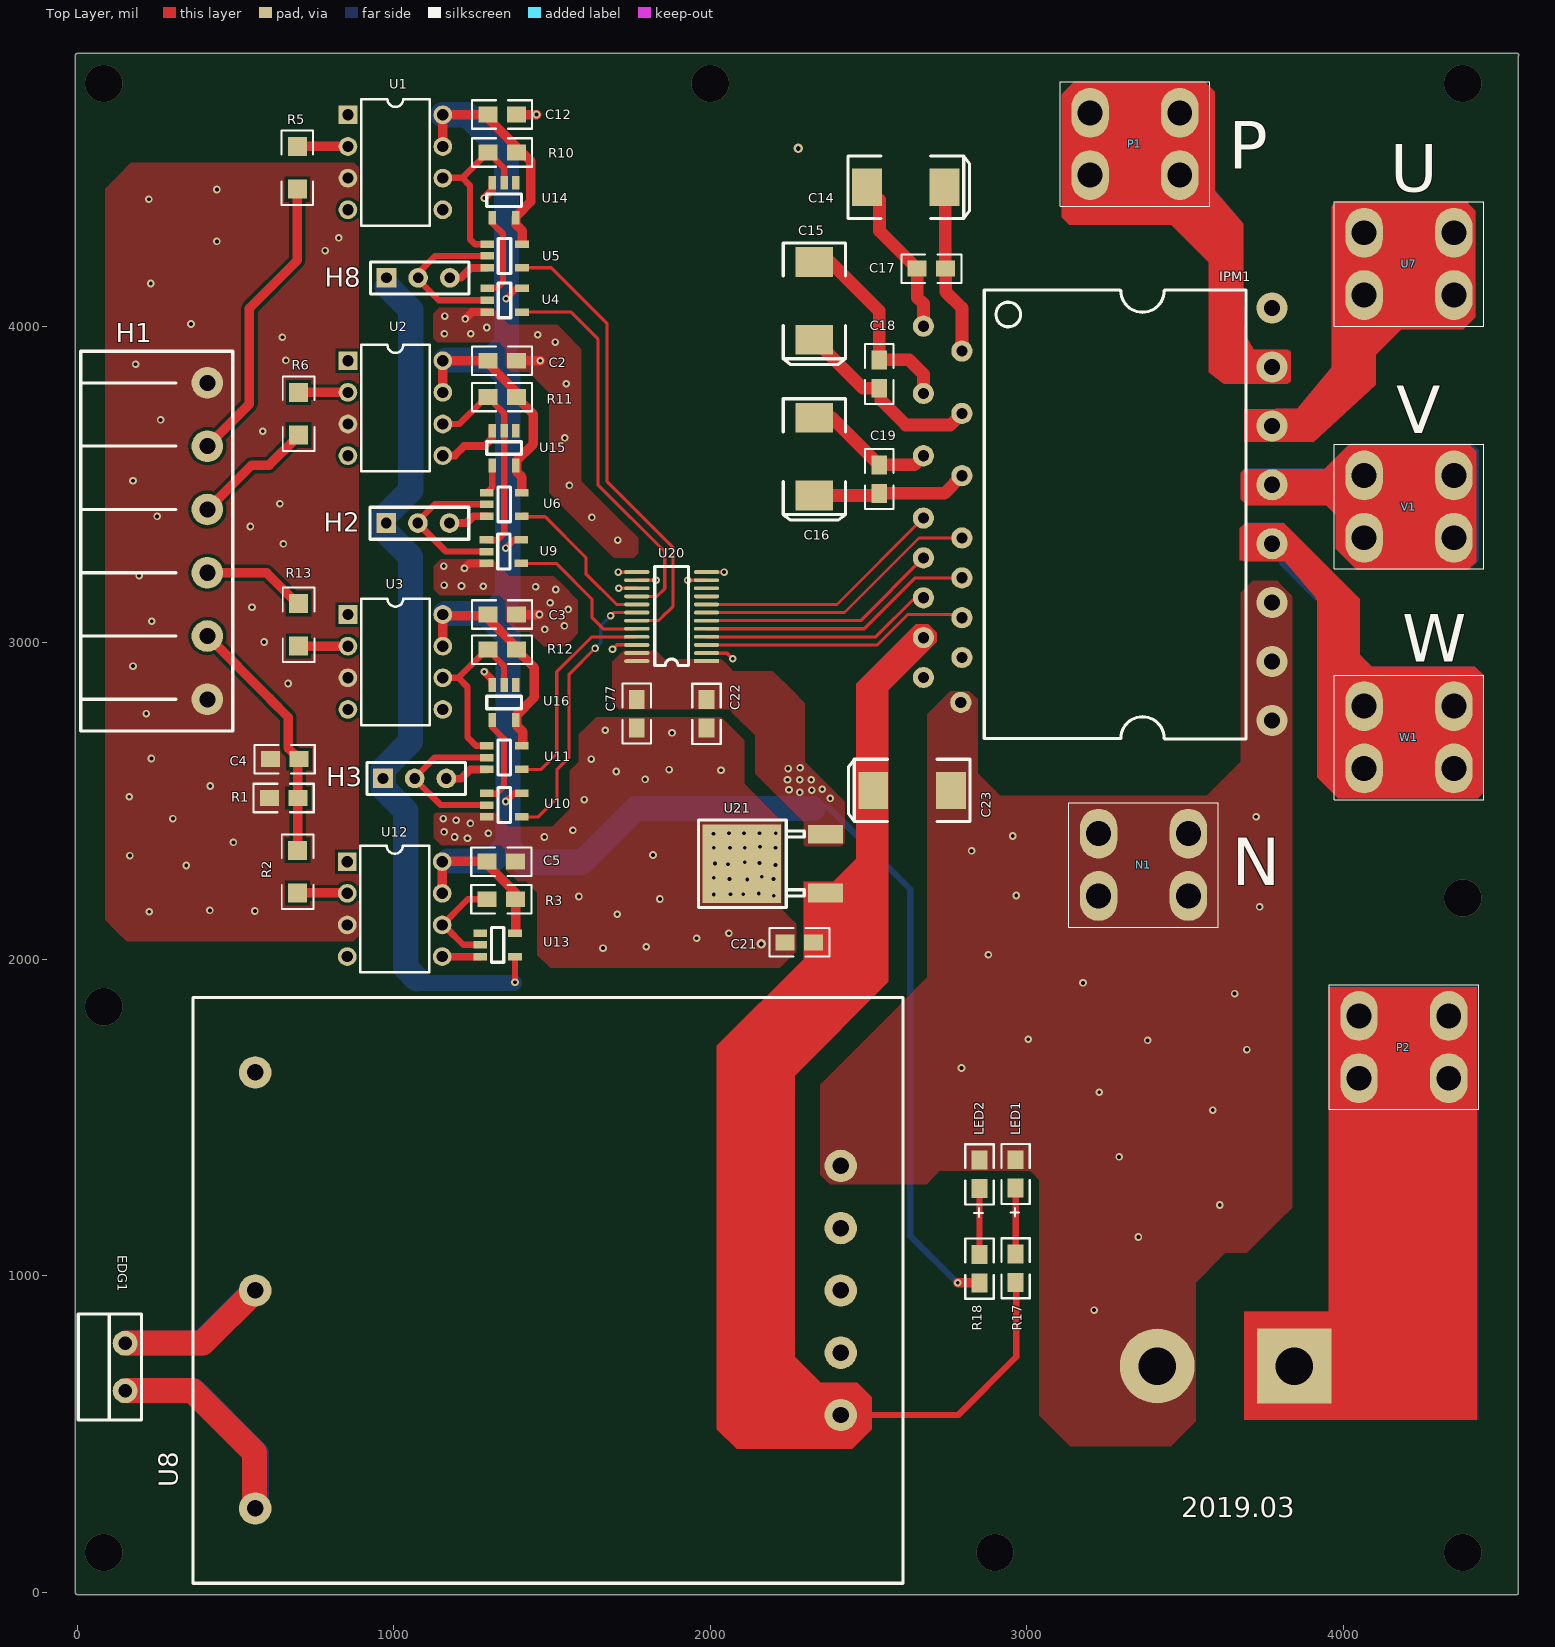
[diagram p0: Top Layer view]
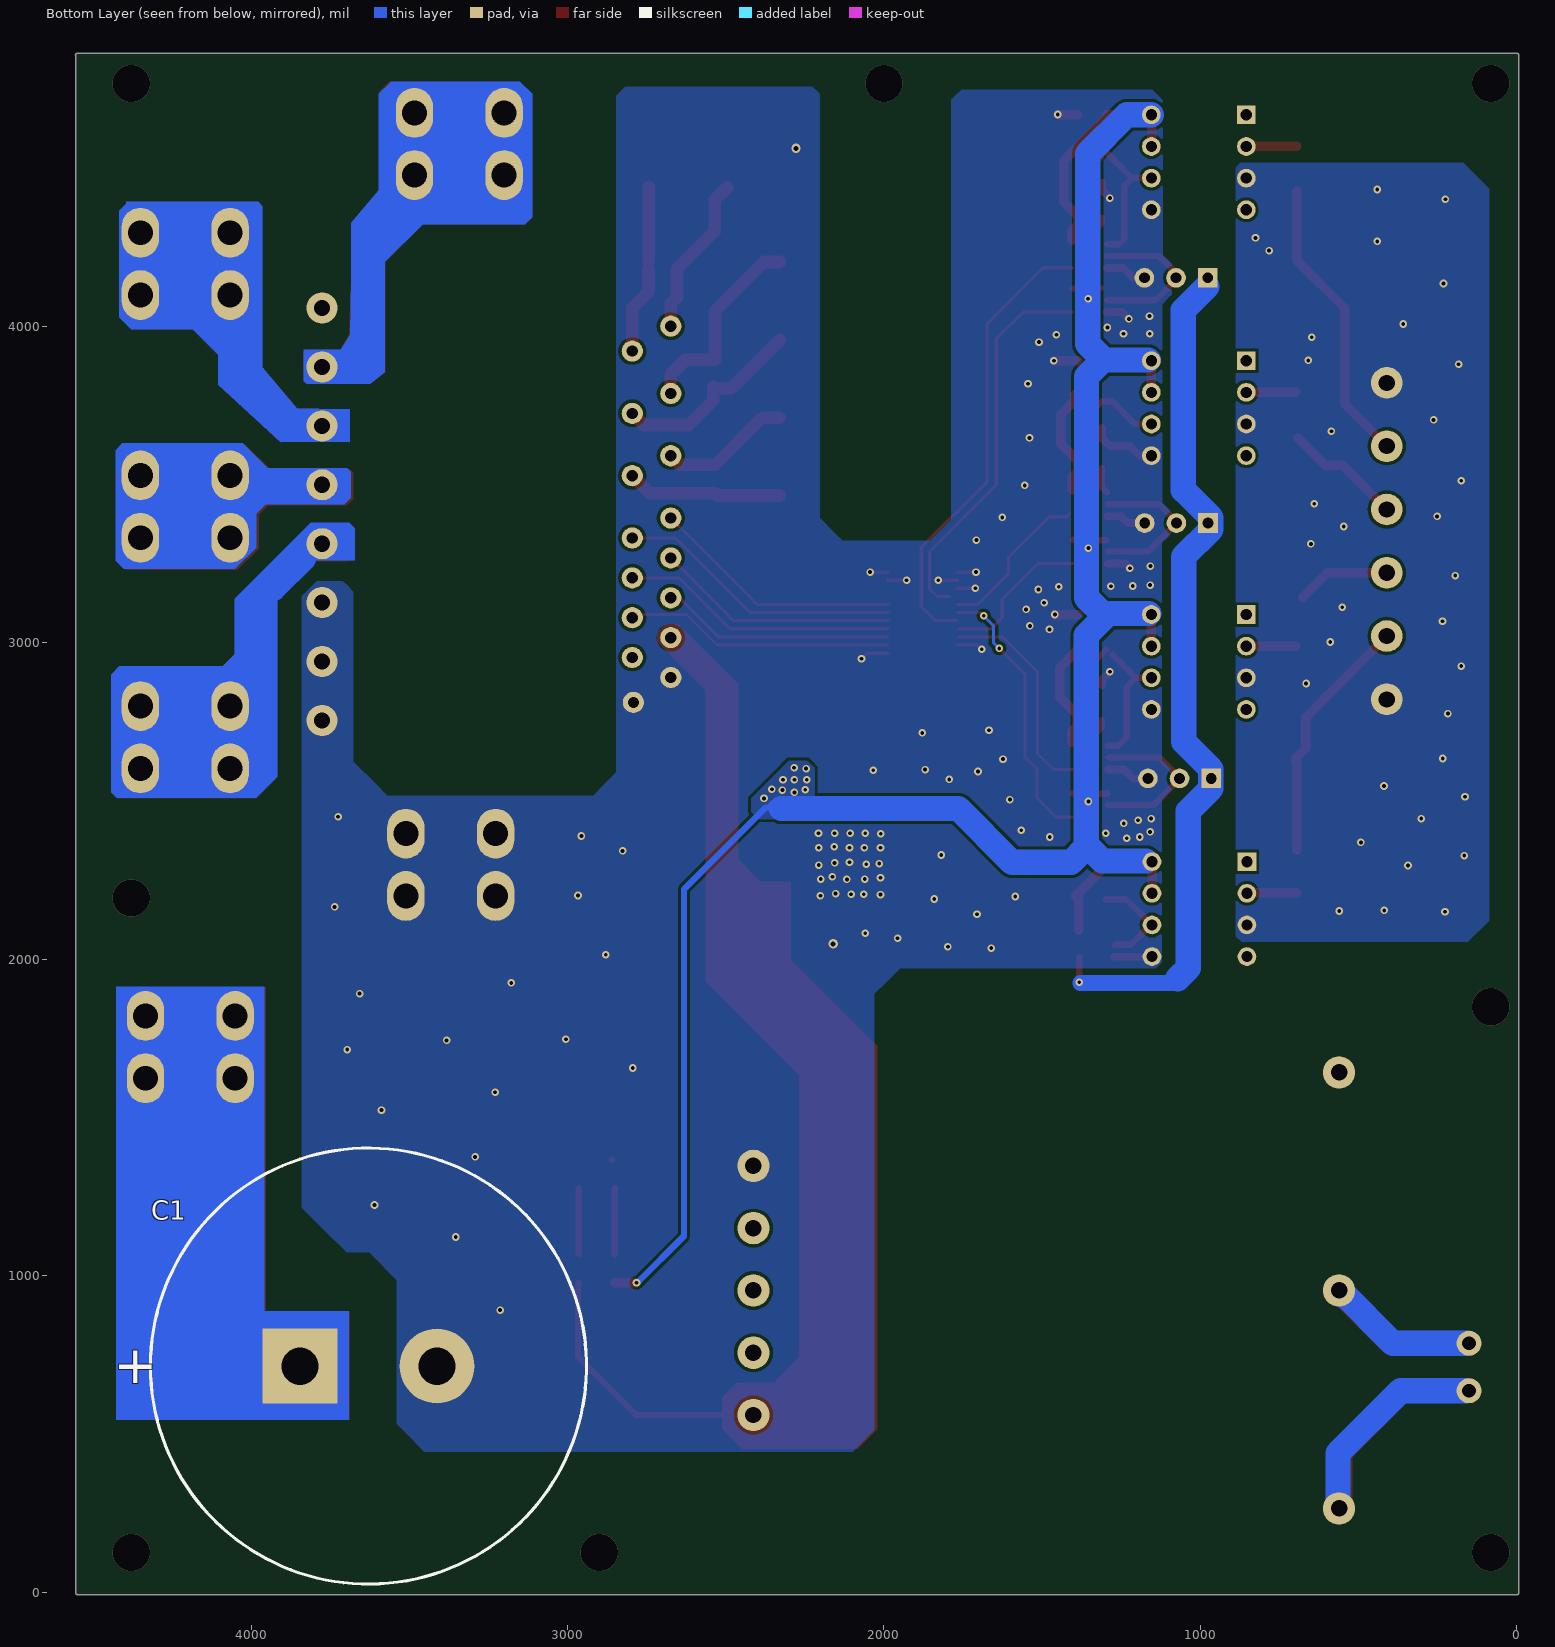
[diagram p1: Bottom Layer view, seen from below]
# Altium PCB MISC81124.PcbDoc
Units mil, origin at the board's own origin, x right, y up, seen from the top; angles counter-clockwise.
Board outline 4561.03 x 4870.03 mil, 2 copper layers (Top Layer, Bottom Layer); 58 components, 50 nets, 240 pads, 164 vias.

## Layer stack, top to bottom (the 12.6 mil dielectric is the usual default, probably not edited)
Top Layer: signal copper 1.4
Dielectric: dielectric 12.6, FR-4, Dk 4.8
Bottom Layer: signal copper 1.4

## Board outline
-6.01,-3 ccw(c-1,-3) -1,-8.01 4547,-8.01 ccw(c4547,-3) 4548,-7.91 ccw(c4549,-3) 4554.01,-3 4554.01,4853.99 ccw(c4550,4857) 4555.01,4857 ccw(c4550,4857) 4550,4862.02 -1,4862.02 ccw(c-1,4857) -6.01,4857

## Design rules (kind name [scope] priority, off if disabled: settings)
Clearance [All] p1: gap=10
ComponentClearance [All] p1 off: gap=10 collisioncheckmode=3 verticalgap=10 showdistances=FALSE
FabricationTestPointUsage TestPointUsage [All] p1: valid=0 allowmultiple=FALSE
FabricationTestpoint Testpoint [(IsPad And (OnTopLayer Or OnBottomLayer))] p1: side=3 testpointundercomponent=TRUE minsize=40 maxsize=100 preferedsize=60 minholesize=0 maxholesize=40 preferedholesize=32 testpointgrid=1 allowsidetop=TRUE allowsidebottom=TRUE usegrid=TRUE gridtolerance=0.01
FanoutControl Fanout_LCC [All] p1 off: bgadir=Out bgaviamode=Centered fanoutstyle=Auto fanoutdirection=Alternating viagrid=1 // Protel DXP Scope 1 Expression Was: IsLCC   Fanout_LCC (Default Rule)
FanoutControl Fanout_BGA [All] p2 off: bgadir=Out bgaviamode=Centered fanoutstyle=Auto fanoutdirection=Alternating viagrid=1 // Protel DXP Scope 1 Expression Was: IsBGA   Fanout_BGA (Default Rule)
FanoutControl Fanout_SOIC [All] p3 off: bgadir=Out bgaviamode=Centered fanoutstyle=Auto fanoutdirection=Alternating viagrid=1 // Protel DXP Scope 1 Expression Was: IsSOIC   Fanout_SOIC (Default Rule)
FanoutControl Fanout_Default [All] p4: bgadir=Out bgaviamode=Centered fanoutstyle=Auto fanoutdirection=Alternating viagrid=1 // Fanout_Default (Default Rule)
FanoutControl Fanout_Small [All] p5 off: bgadir=Out bgaviamode=Centered fanoutstyle=Auto fanoutdirection=Alternating viagrid=1 // Protel DXP Scope 1 Expression Was: (CompPinCount < 5)   Fanout_Small (Default Rule)
Height [All] p1 off: minheight=0 maxheight=1000 prefheight=500
HoleSize [All] p1: absolutevalues=TRUE maxlimit=150 minlimit=6 maxpercent=80.000 minpercent=20.000
MinimumSolderMaskSliver [All] p1: minsoldermaskwidth=0
PlaneConnect [All] p1: planeconnectstyle=Direct reliefexpansion=20 reliefentries=4 reliefconductorwidth=10 reliefairgap=10
PolygonConnect [All] p1: connectstyle=Direct reliefconductorwidth=75 reliefentries=4 polygonreliefangle="90 Angle"
RoutingVias [All] p1: holewidth=12 width=24 viastyle="Through Hole" minholewidth=12 minwidth=24 maxholewidth=12 maxwidth=24
SilkToSilkClearance [All] p1: silktosilkclearance=0
SilkscreenOverComponentPads [IsPad] p1 off: minsilkscreentomaskgap=10 // Protel DXP Scope 1 Expression Was: IsPad
SolderMaskExpansion [All] p1: expansion=4
Width [All] p1: maxlimit=99 minlimit=10 preferedwidth=11.81
14 further rules are at their usual default settings.

## Components (designator, comment, footprint, x,y, rotation, side; value= is the part's Value field where it differs from the comment)
C1 "450V" ElecCap_450V 3629,714 r180 bottom
C2 "0.1uF" 0805 1387,3891 r180 top
C3 "0.1uF" 0805 1387,3089 r180 top
C4 "30pF" 0805 610,2632 r0 top
C5 "0.1uF" 0805 1385,2308 r180 top
C12 "0.1uF" 0805 1387,4669 r180 top
C14 "22uF/35V" 7343_CASE-D 2618,4439 r0 top
C15 "22uF/35V" 7343_CASE-D 2329,4080 r270 top
C16 "22uF/35V" 7343_CASE-D 2329,3588 r270 top
C17 "0.1uF" 0805 2744,4182 r180 top
C18 "0.1uF" 0805 2534,3804 r90 top
C19 "0.1uF" 0805 2534,3472 r90 top
C21 "0.33uF" 0805 2237,2053 r0 top
C22 "0.01uF" 0805 1988,2730 r90 top
C23 "22uF/35V" 7343_CASE-D 2638,2533 r180 top
C77 "0.1uF" 0805 1768,2821 r270 top
EDG1 "EDG 2p" EDGCon_2p_3.81mm 151,786 r270 top
H1 "Header6" EDGCon_6P_5.08mm 411,3821 r270 top
H2 "Header3" PinHeader3_2.54mm 976,3378 r0 top
H3 "Header3" PinHeader3_2.54mm 966,2571 r0 top
H8 "Header3" PinHeader3_2.54mm 977,4153 r0 top
IPM1 "IKCM15F60GA" IKCM15F60GA 3692.77,2697 r90 top
LED1 "LED" 0805_LED 2965,1276 r90 top
LED2 "LED" 0805_LED 2851,1275 r90 top
N1 "PCBTerminator" PCBTerminator 3369,2298 r90 top
P1 "PCBTerminator" PCBTerminator 3342,4576 r90 top
P2 "PCBTerminator" PCBTerminator 4192,1722 r90 top
R1 "10k" 0805 607,2509 r0 top
R2 "500R" 1206 696,2209 r90 top
R3 "10k" 0805 1295,2189 r0 top
R5 "500R" 1206 695,4568 r270 top
R6 "500R" 1206 699,3791 r270 top
R10 "10k" 0805 1297,4549 r0 top
R11 "10k" 0805 1297,3776 r0 top
R12 "10k" 0805 1297,2978 r0 top
R13 "500R" 1206 699,2989 r90 top
R17 "10k" 0805 2965,1068 r270 top
R18 "3.3k" 0805 2851,1067 r270 top
U1 "6N137" DIP-8 855,4668 r0 top
U2 "6N137" DIP-8 855,3891 r0 top
U3 "6N137" DIP-8 855,3089 r0 top
U4 "SN74AHC1G08" SOT-23-5 1350,4082 r180 top
U5 "SN74AHC1G08" SOT-23-5 1350,4222 r180 top
U6 "SN74AHC1G08" SOT-23-5 1349,3437 r180 top
U7 "PCBTerminator" PCBTerminator 4208,4197 r90 top
U8 "YAS5-15-W" YAS5 1487.2,953.02 r180 top
U9 "SN74AHC1G08" SOT-23-5 1348,3288 r180 top
U10 "SN74AHC1G08" SOT-23-5 1349,2487 r180 top
U11 "SN74AHC1G08" SOT-23-5 1349,2637 r180 top
U12 "6N137" DIP-8 853,2308 r0 top
U13 "SN74AHC1G04" SOT-23-5 1328,2045 r180 top
U14 "SN74AHC1G04" SOT-23-5 1348.65,4398 r90 top
U15 "SN74AHC1G04" SOT-23-5 1348.65,3615 r90 top
U16 "SN74AHC1G04" SOT-23-5 1348.65,2811 r90 top
U20 "SN74LVC8T245" SN74LVC8T245_TSSOP24 1988,3223.13 r180 top
U21 "L78M05" TO-252-2(DPAK) 2364,2302 r0 top
V1 "PCBTerminator" PCBTerminator 4208,3430 r90 top
W1 "PCBTerminator" PCBTerminator 4208,2701 r90 top

## Footprints (in the part's own frame and the unit in brackets; to place one, negate y for a bottom-side part, rotate by r counter-clockwise, add the part's x,y. Pads: shape width x height; smd on the part's side, far side on the other; paste and mask are expansions set on the pad)
0805 [mil]
  rect 60x50 smd: 1(0,0) 2(90,0)
  silkscreen extent -50,-45 140,45
0805_LED [mil]
  rect 60x50 smd: A(0,0) K(90,0)
  silkscreen extent -90,-45 140,45
1206 [mil]
  rect 60x60 smd: 1(0,0) 2(135,0)
  silkscreen extent -50,-50 185,50
7343_CASE-D [mm]
  rect 2.4x3 smd: 1(3.12,0) 2(-3.12,0)
  silkscreen extent -4.65,-2.5 5.1,2.5
DIP-8 [mm]
  rect 1.5x1.5 hole 0.9: 1(0,0)
  round 1.5 hole 0.9: 2(0,-2.54) 3(0,-5.08) 4(0,-7.62) 5(7.62,-7.62) 6(7.62,-5.08) 7(7.62,-2.54) 8(7.62,0)
  silkscreen extent 1.06,-8.88 6.56,1.27
EDGCon_2p_3.81mm [mm]
  round 2 hole 1.1: 1(0,0) 2(3.81,0)
  silkscreen extent -2.34,-3.76 6.15,1.32
EDGCon_6P_5.08mm [mil]
  round 100 hole 51: 1(0,0) 2(200,0) 3(400,0) 4(600,0) 5(800,0) 6(1000,0)
  silkscreen extent -100,-400 1100,80
ElecCap_450V [mm] "820"
  rect 6x6 hole 3: 1(-5.5,0)
  round 6 hole 3: 2(5.5,0)
  silkscreen extent -17.5,-17.5 17.5,17.5
IKCM15F60GA [mm] "Infineon IPM"
  round 1.7 hole 0.9: 1(33.1,25.885) 2(31.1,22.793) 3(27.7,25.885) 4(26.1,22.793) 5(22.7,25.885) 6(21.1,22.793) 7(17.7,25.885) 8(16.1,22.793) 9(14.5,25.885) 10(12.9,22.793) 11(11.3,25.885) 12(9.7,22.793) 13(8.1,25.885) 14(6.507,22.793) 15(4.9,25.885) 16(2.9,22.885)
  round 2.5 hole 1.3: 17(1.45,-2.1) 18(6.18,-2.1) 19(10.91,-2.1) 20(15.64,-2.1) 21(20.37,-2.1) 22(25.1,-2.1) 23(29.83,-2.1) 24(34.56,-2.1)
  silkscreen extent -0.03,0 36,21
PCBTerminator [mm]
  oval 4x3 hole 2: 1(-2.5,3.6) 1(-2.5,-3.6) 1(2.5,3.6) 1(2.5,-3.6)
  silkscreen extent -5,-6 5,6
PinHeader3_2.54mm [mil]
  rect 62x62 hole 34: 1(0,0)
  round 62 hole 34: 2(100,0) 3(200,0)
  silkscreen extent -51,-51 261,50
SN74LVC8T245_TSSOP24 [mil]
  rect 80x12 smd: 1(0,281.49)
  oval 80x12 smd: 2(0,255.9) 3(0,230.31) 4(0,204.72) 5(0,179.13) 6(0,153.54) 7(0,127.95) 8(0,102.36) 9(0,76.77) 10(0,51.18) 11(0,25.59) 12(0,0) 13(220,0) 14(220,25.59) 15(220,51.18) 16(220,76.77) 17(220,102.36) 18(220,127.95) 19(220,153.54) 20(220,179.13) 21(220,204.72) 22(220,230.31) 23(220,255.9) 24(220,281.49)
  silkscreen extent 56,-18 163,295
SOT-23-5 [mm]
  rect 1.1x0.6 smd: 1(1.4,-0.95) 2(1.4,0) 3(1.4,0.95) 4(-1.4,0.95) 5(-1.4,-0.95)
  silkscreen extent -0.5,-1.4 0.5,1.4
TO-252-2(DPAK) [mm]
  rect 6.3x6.3 smd: 1(-6.7,0)
  rect 2.8x1.5 smd: 2(-0.004,2.361) 3(0,-2.361)
  silkscreen extent -10.2,-3.52 -1.7,3.5
YAS5 [mm]
  round 2.6 hole 1.321: 1(23.5,17.5) 2(23.5,0) 3(23.5,-17.5) 4(-23.5,-10) 5(-23.5,-5) 6(-23.5,0) 7(-23.5,5) 8(-23.5,10)
  silkscreen extent -28.5,-23.5 28.5,23.5

## Part data
C1: library part ELECTROCap, "Electrolytic Capacitor(Pin1 Positive)"
C2 C3 C4 C5 C12 C17 C18 C19 C21 C22 C77: library part CAP, "Capacitor"
C14 C15 C16 C23: library part TaCap_D, "TaCap_D"
N1 P1 P2 U7 V1 W1: "PCB terminal for high current"
R1 R2 R3 R5 R6 R10 R11 R12 R13 R17 R18: library part RES2
U1 U2 U3 U12: "High-speed optocoupler"
U4 U5 U6: "Single 2-Input Positive-AND Buffer"
U8: library part YAS5
U9 U10 U11 U13 U14 U15 U16: "Single Input Inverter"
U20: "TI SN74LVC8T245PWR"
U21: library part LM1085ISX-3.3

## Via types
v1: diameter 24, hole 12, Top Layer to Bottom Layer, 154 vias
v2: diameter 118.11, hole 118.11, Top Layer to Bottom Layer, 8 vias
v3: diameter 30, hole 15, Top Layer to Bottom Layer, tented both sides, 2 vias

## Nets (pads, with @x,y where several pads share a name; then routed paths per layer and width w, separated by ;. In a path a pad name is that pad's centre, name@x,y a point inside that pad or via, vN(x,y) a via of type N, cw(c..) or ccw(c..) an arc to the next point about the centre after c; other vN are vias at no path point)
+5V_IPM: C2.2 C3.2 C5.2 C12.2 C22.2 C77.1 R3.2 R10.2 R11.2 R12.2 R18.2 U1.7 U1.8 U2.7 U2.8 U3.7 U3.8 U4.5 U5.5 U6.5 U9.5 U10.5 U11.5 U12.7 U12.8 U13.5 U14.5 U15.5 U16.5 U20.1 U20.23 U20.24 U21.2 | length 8699.7
  Top Layer w20: v1(1354,2498) 1380.4,2524.4 U10.5 ; v1(1354,3299) 1380.4,3325.4 U9.5 ; v1(1355,4087) 1387.4,4119.4 U4.5
  Top Layer w30: U12.7 U12.8 1153,2310 1293,2310 1297,2306 1297,2297 R3.2@1395,2199 ; U1.7@1154,4579 1154,4662 1164,4672 1167,4669 C12.2 C12.2@1297,4668.64 ; U3.7 1155,3082 1158,3085 C3.2@1283,3085 ; U2.7 U2.8@1155,3884 ; U2.8@1160,3891 C2.2 1297,3883 R11.2@1398,3782 ; C3.2@1283,3083 1291,3083 1387,2987 R12.2 1444,2921 1444,2827 1389,2772 1389,2737 1407,2719 U11.5@1407,2686 ; C12.2@1289,4668 1289,4666 1432.5,4522.5 1432.5,4393.5 U14.5@1392,4353 ; U13.5@1385,2091 R3.2 ; U14.5 1386.06,4321.94 1406,4302 1406,4272 ; R11.2 1441,3722 1441,3628 1388,3575 1388,3540 1405,3523 U6.5@1405,3484 ; v1(2782,977) R18.2
  Bottom Layer w20: 2345,2479 2374,2479 2632,2221 2632,1125 v1@2780,977
  Bottom Layer w50: U12.8@1157,2310 U12.8@1172,2310 ; U3.8@1160,3090 U3.8@1163,3090 ; U2.8@1160,3893 U2.8@1165,3893 ; 2325,2480 2343,2480
  Bottom Layer w80: U1.8 1233,4668 1356,4545 1356,3944 1305,3893 U2.8@1165,3893 ; U3.8@1163,3092 1292,3092 1361,3023 1361,2409 1361,2354 1409,2306 1595,2306 1765,2476 2325,2476 ; U12.8@1172,2310 1310,2310 1359,2359 ; 1308,3893 1360,3841 1360,3142 1310,3092
  other v1: 2379,2508 2283,2527 2321,2534 2249,2535 2354,2537 2244,2567 2283,2567 2319,2567 2246,2602 2284,2605
+15V_IPM: C21.2 C23.1 IPM1.13 R17.2 U8.8 U21.3 | length 1600.4
  Top Layer w20: U8.8@2421.07,568 U8.8 2783.32,559.32 2967,743 R17.2@2967,970 ; R17.2@2962,975 R17.2
  Top Layer w50: 2499,2362 2499,2841.24 IPM1.13
AC1: EDG1.2 U8.1 | length 1282.8
  Top Layer w80: EDG1.2@157,637 364,637 560,441 U8.1@560,265
  Bottom Layer w80: EDG1.2@161,636 368,636 565,439 U8.1@565,302
AC2: EDG1.1 U8.2 | length 940.7
  Top Layer w80: EDG1.1@155,787 392,787 ; 396,787 U8.2@561,952
  Bottom Layer w80: EDG1.1@154,786 391,786 U8.2@556,951
GND: C4.1 H1.1 H1.6 R1.1 U1.3 U2.3 U3.3 U12.3
  other v1: 227,2150 561,2152 419,2154 344,2296 166,2327 493,2369 302,2444 164,2513 420,2547 234,2634 218,2776 666,2871 176,2926 590,3002 235,3068 552,3112 195,3212 651,3312 547,3367 252,3399 640,3439 176,3512 586,3668 263,3704 184,3880 659,3892 648,3965 359,4007 232,4135 783,4239 441,4268 826,4279 226,4401 441,4432
IPM_N: C1.2 C2.1 C3.1 C5.1 C12.1 C21.1 C22.1 C23.2 C77.2 H2.3 H3.3 H8.3 IPM1.15 IPM1.16 IPM1.17 IPM1.18 IPM1.19 LED1.K LED2.K N1.1 U1.5 U2.5 U3.5 U4.3 U5.3 U6.3 U8.4 U9.3 U10.3 U11.3 U12.5 U13.3 U14.3 U15.3 U16.3 U20.2 U20.11 U20.12 U20.13 U20.14 U20.15 U20.22 U21.1 | length 1692.9
  Top Layer w11: v1(1691,2979) 1704.82,2992.82 U20.22 ; v1(1709.13,3223.13) U20.13 ; v1(1710.95,3171.95) U20.15 ; U20.14 v1(1828.46,3197.54) ; v1(1928.54,3197.54) U20.11 ; U20.2 2052.77,2967.23 v1(2071,2949) ; U20.12 v1(2043.87,3223.13)
  Top Layer w20: LED2.K@2858,1366 LED2.K@2859,1365
  Top Layer w25: U2.5@1142,3592 1193,3592 1222,3621 1286,3621 1311.25,3646.25 U15.3 ; H3.3@1148,2570 1212,2570 1241.6,2599.6 U11.3 ; U12.5@1164.4,2007.6 U13.3 ; H8.3@1173,4154 1213,4154 1243.6,4184.6 U5.3 ; H2.3@1174,3378 1230,3378 1251.6,3399.6 U6.3 ; v1(1223,3235) 1238.6,3250.6 U9.3 ; v1(1226,4023) 1247.6,4044.6 U4.3 ; v1(1286,2908) 1311.25,2882.75 U16.3 ; v1(1286,4405) 1311.25,4430.25 U14.3 ; U15.3@1311,3678 U15.3@1311.25,3677.75
  Top Layer w30: C3.1 v1(1460,3089) ; C2.1 v1(1463,3891) ; C12.1 v1(1451,4669)
  Bottom Layer w60: IPM1.15 IPM1.15@2676.09,2889.91
  other v1: 3213,891 3353,1122 3610,1223 3292,1375 3588,1523 3229,1579 2794,1656 3696,1714 3382,1743 3005,1747 3657,1891 3178,1925 2879,2014 1661,2035 1798,2039 1957,2066 2059,2082 1706,2142 3736,2165 1841,2190 1585,2198 2201,2200 2967,2201 2011,2204 2064,2205 2104,2205 2153,2207 2117,2252 2061,2253 2200,2253 2011,2257 2163,2260 2206,2297 2056,2300 2015,2302 2156,2304 2109,2306 1819,2329 2826,2342 2011,2352 2062,2352 2109,2352 2206,2352 2157,2355 1233,2382 1192,2386 1476,2386 2956,2389 2010,2396 1299,2398 2059,2398 2107,2398 2156,2398 2207,2398 1159,2402 1566,2407 1242,2429 1197,2439 1156,2444 3725,2450 1602,2504 1794,2568 1703,2593 2034,2597 1870,2599 1624,2632 1879,2715 1668,2723 1477,3042 1539,3053 1551,3105 1494,3126 1512,3168 1448,3177 1283,3178 1214,3179 1159,3182 1158,3242 1708,3324 1626,3396 1555,3497 1540,3647 1545,3818 1510,3950 1455,3973 1160,3976 1243,3976 1294,3996 1161,4032
  other v3: 2161,2048 2278,4562
IPM_P: IPM1.23 P1.1
IPM_U: IPM1.22 U7.1
IPM_V: IPM1.21 V1.1
IPM_W: IPM1.20 W1.1 | length 161.2
  Top Layer w10: 3918,3138 3918,3155
  Bottom Layer w40: 3816,3257 3918,3155
NetC1_1: C1.1 P2.1
NetC14_1: C14.1 C17.1 IPM1.2 | length 516
  Top Layer w40: C17.1@2742.83,4206.83 C14.1@2742.83,4441 ; C17.1 2744,4109 2795.4,4057.6 IPM1.2
NetC14_2: C14.2 C17.2 IPM1.1 | length 512.8
  Top Layer w40: C14.2 2535,4399.17 2535,4301 C17.2 2654,4091 2673.66,4071.34 IPM1.1
NetC15_1: C15.1 C18.1 IPM1.4 | length 614.7
  Top Layer w40: C15.1 2482.17,3804 C18.1 ; C18.1@2539,3809 2539,3767 2618,3688 2758.84,3688 IPM1.4
NetC15_2: C15.2 C18.2 IPM1.3 | length 642.5
  Top Layer w40: C15.2 2379.17,4202.83 2534,4048 C18.2 2628,3894 2673.66,3848.34 IPM1.3
NetC16_1: C16.1 C19.1 IPM1.6 | length 492.3
  Top Layer w40: C16.1 2527.17,3465.17 C19.1 2739.69,3472 IPM1.6
NetC16_2: C16.2 C19.2 IPM1.5 | length 418.2
  Top Layer w40: C16.2 2385.17,3710.83 C19.2 2644.96,3562 IPM1.5
NetLED1_A: LED1.A R17.1 | length 208
  Top Layer w20: R17.1 LED1.A
NetLED2_A: LED2.A R18.1 | length 210.8
  Top Layer w20: LED2.A@2849,1277 LED2.A R18.1
NetR2_1: R2.1 U12.2 | length 152
  Top Layer w30: R2.1 U12.2@848,2209
NetR3_1: R3.1 U12.6 U13.2 | length 309.2
  Top Layer w20: U12.6 1234,2189 R3.1 R3.1@1300,2189 ; U12.6@1165,2100 1220,2045 U13.2@1270.88,2045
NetR5_1: R5.1 U1.2 | length 158.1
  Top Layer w30: R5.1 846,4568 U1.2@851,4563
NetR6_1: R6.1 U2.2 | length 137
  Top Layer w30: R6.1 U2.2@836,3791
NetR10_1: R10.1 U1.6 U5.1 U14.2 | length 536.5
  Top Layer w20: U1.6@1155,4469 1216,4469 ; U5.1 1256.6,4259.4 1241,4275 1241,4444 1216,4469 ; R10.1 1217,4469 1216,4469 ; R10.1@1313,4535 1348.65,4499.35 U14.2
NetR11_1: R11.1 U2.6 U9.1 U15.2 | length 678.8
  Top Layer w20: U2.6 1207,3691 1279,3763 1310,3763 1348.65,3724.35 U15.2 1348.65,3345.65 1327,3324 U9.1@1297,3324
NetR12_1: R12.1 U3.6 U11.1 U16.2 | length 540.4
  Top Layer w20: U3.6 1204,2889 R12.1@1277,2962 ; 1206,2887 1233,2860 1233,2701 1259.6,2674.4 U11.1 ; R12.1 1348,2927 1348,2894 U16.2@1348,2880
NetR13_1: R13.1 U3.2 | length 145
  Top Layer w30: R13.1 U3.2@844,2989
NetU4_1: U4.1 U14.4 | length 254.7
  Top Layer w20: U14.4 1311.25,4325.75 1345,4292 1345,4140 1326,4121 U4.1@1315,4121
NetU6_1: U6.1 U15.4 | length 83.7
  Top Layer w20: U6.1 1311,3491.52 U15.4@1311,3551
NetU10_1: U10.1 U16.4 | length 289
  Top Layer w20: U10.1@1293,2523 1324,2523 1348,2547 1348,2696 1311.25,2732.75 U16.4
PWM_UH: U4.4 U20.16 | length 1225.7
  Top Layer w10: U4.4 1560.4,4044.6 1645,3960 1645,3499 1856,3288 1856,3171 1831,3146 U20.16@1792,3146
PWM_UL: U5.4 U20.19 | length 1454.3
  Top Layer w10: U5.4 1497.4,4184.6 1674,4008 1674,3509 1882,3301 1882,3114 1862,3094 ; U20.19 1836.59,3069.59 1861.5,3094.5
PWM_VH: U6.4 U20.17 | length 502.4
  Top Layer w10: U6.4@1414,3407 1423,3398 1478,3398 1607,3269 1607,3218 1704.23,3120.77 U20.17
PWM_VL: U9.4 U20.20 | length 507.5
  Top Layer w10: U9.4@1393,3251 1393.4,3250.6 U9.4 1480,3250.6 ; 1498.4,3250.6 1480,3250.6 ; U20.20@1762,3043 1663,3043 1626,3080 1626,3138 1513.4,3250.6 1480,3250.6
PWM_WH: U10.4 U20.18 | length 867.3
  Top Layer w10: U10.4 1456.6,2449.6 1516,2509 1516,2600 1554,2638 1554,2900 v1(1636,2982) ; v1(1685,3085) 1695.18,3095.18 U20.18
  Bottom Layer w10: v1(1636,2982) 1654,3000 1654,3053 v1@1684,3083
PWM_WL: U11.4 U20.21 | length 682.9
  Top Layer w10: U11.4 1465.6,2599.6 1515,2649 1515,2908 1625,3018 U20.21@1762,3018
PWMEN: H2.1 H3.1 H8.1 U13.4 | length 2757.6
  Top Layer w20: v1(1383.12,1927.12) U13.4
  Bottom Layer w50: 1072,1925 v1@1380,1925
  Bottom Layer w80: H8.1@979.5,4125.5 1054,4051 1054,3482 967,3395 967,3358 1053,3272 1053,2687 967,2601 967,2539 1038,2468 1038,1972 1072,1938
PWMEN_IN: C4.2 H1.5 R1.2 R2.2 | length 806.2
  Top Layer w30: H1.5 609.5,2822.5 ; 609,2822 666.5,2764.5 666.5,2666.5 C4.2@696,2637 ; R2.2 C4.2@696,2637 ; C4.2@697,2636 C4.2@696,2637 ; C4.2@698,2626 C4.2@698,2636
PWMUEN: H8.2 U4.2 U5.2 | length 508.5
  Top Layer w10: U5.2@1294,4222 U5.2
  Top Layer w20: U5.2@1294,4222 1131,4222 1074,4165 1074,4150 1142,4082 U4.2
PWMUH: IPM1.7 U20.8 | length 798.8
  Top Layer w10: U20.8 2400.58,3120.77 IPM1.7
PWMUH_IN: H1.2 R5.2 | length 922.6
  Top Layer w30: H1.2 544,3754 544,4057 695,4208 R5.2@695,4426
PWMUL: IPM1.10 U20.5 | length 874
  Top Layer w10: U20.5 2487,3044 2647.87,3204.87 IPM1.10
PWMVEN: H2.2 U6.2 U9.2 | length 495.2
  Top Layer w20: H2.2@1075,3375 H2.2@1075,3388 ; H2.2@1078,3375 1165,3288 U9.2 ; H2.2@1081,3388 1130,3437 U6.2@1292,3437
PWMVH: IPM1.8 U20.7 | length 905
  Top Layer w10: U20.7 2424.18,3095.18 2659.86,3330.86 IPM1.8
PWMVH_IN: H1.3 R6.2 | length 374.6
  Top Layer w30: H1.3 551,3561 606,3561 R6.2@692,3647
PWMVL: IPM1.11 U20.4 | length 736.8
  Top Layer w10: U20.4 2523.41,3018.41 2646.88,3141.88 IPM1.11
PWMWEN: H3.2 U10.2 U11.2 | length 492.9
  Top Layer w10: U11.2@1289,2637 U11.2@1296,2637
  Top Layer w20: H3.2@1074,2581 1130,2637 U11.2@1289,2637 ; H3.2@1076,2559 1148,2487 U10.2
PWMWH: IPM1.9 U20.6 | length 767.8
  Top Layer w10: U20.6 2475.39,3069.59 IPM1.9
PWMWH_IN: H1.4 R13.2 | length 298.7
  Top Layer w30: H1.4 598,3221 R13.2@677,3142
PWMWL: IPM1.12 U20.3 | length 851.4
  Top Layer w10: U20.3 2527.82,2992.82 2624,3089 2785.29,3089 IPM1.12
pads on no net: IPM1.14 IPM1.24 U1.1 U1.4 U2.1 U2.4 U3.1 U3.4 U8.3 U8.5 U8.6 U8.7 U12.1 U12.4 U13.1 U14.1 U15.1 U16.1 U20.9 U20.10
copper on no net:
  other v2: 83,125 2900,125 4378.28,125 83,1849 4378.28,2193 83,4767 2000,4767 4378.28,4767

## Polygon pours and split planes (outlines as drawn)
+5V_IPM on Top Layer "Top Layer-No Net" (solid, remove dead copper, pour order 1000): 2295,2417 2295,2369 2295,2362 2297,2360 2301,2356 2314,2356 2414,2356 2421,2363 2425,2367 2425,2378 2425,2497 2367,2555 2299,2623 2299,2735 2299,2809 2259,2849 2198,2910 2074,2910 2073,2910 2050,2933 2035,2948 2019,2948 1856,2948 1841,2963 1829,2975 1792,2975 1726,2975 1713,2962 1690,2939 1690,2900 1690,2812 1698,2804 1713,2789 1760,2789 2060,2789 2078,2771 2142,2707 2142,2676 2142,2586 2221,2507 2295,2433 2295,2417
GND on Top Layer "Top Layer-No Net" (solid, remove dead copper, pour order 1001): 88,4346 88,4255 88,2124 122,2090 156,2056 851,2056 872,2056 882,2066 889,2073 889,2094 889,2136 889,4502 877,4514 875,4516 854,4516 169,4516 127,4474 88,4435 88,4346
IPM_N on Top Layer "Top Layer-No Net" (solid, remove dead copper, pour order 1002): 2347,1479 2347,1319 2369,1297 2377,1289 2443,1289 2684,1289 2710,1315 2726,1331 2835,1331 3010,1331 3020,1321 3039,1302 3039,1257 3039,559 3077,521 3138,460 3218,460 3455,460 3507,512 3534,539 3534,584 3534,978 3618,1062 3628,1072 3647,1072 3696,1072 3794,1170 3839,1215 3839,1247 3839,3147 3805,3181 3791,3195 3771,3195 3714,3195 3699,3180 3676,3157 3676,3140 3676,2623 3574,2521 3569,2516 3506,2516 2917,2516 2876,2557 2845,2588 2845,2630 2845,2821 2830,2836 2819,2847 2797,2847 2759,2847 2731,2819 2686,2774 2686,2562 2686,1942 2521,1777 2347,1603 2347,1479
IPM_N on Top Layer "Top Layer-No Net" (solid, remove dead copper, pour order 1003): 1264,2448 1264,2373 1274,2363 1277,2360 1315,2360 1339,2360 1345,2354 1352,2347 1352,2336 1352,2285 1359,2278 1391,2246 1408,2246 1417,2246 1429,2234 1453,2210 1453,2145 1453,2013 1486,1980 1494,1972 1537,1972 2219,1972 2258,2011 2271,2024 2271,2061 2271,2112 2250,2133 2227,2156 2227,2205 2227,2434 2202,2459 2107,2554 2107,2623 2107,2692 2078,2721 2035,2764 2001,2764 1639,2764 1609,2734 1585,2710 1585,2683 1585,2624 1564,2603 1556,2595 1556,2558 1556,2473 1523,2440 1503,2420 1502,2419 1396,2419 1363,2419 1327,2455 1319,2463 1306,2463 1274,2463 1269,2458 1264,2453 1264,2448
IPM_N on Top Layer "Top Layer-No Net" (solid, remove dead copper, pour order 1004): 1127,2457 1127,2383 1137,2373 1150,2360 1286,2360 1312,2360 1322,2370 1327,2375 1327,2401 1327,2449 1315,2461 1313,2463 1275,2463 1133,2463 1127,2457
IPM_N on Top Layer "Top Layer-No Net" (solid, remove dead copper, pour order 1005): 1124,4040 1124,3969 1124,3963 1130,3957 1138,3949 1189,3949 1333,3949 1345,3937 1354,3928 1354,3912 1354,3872 1360,3866 1370,3856 1405,3856 1425,3856 1440,3841 1491,3790 1491,3698 1491,3539 1491,3473 1567,3397 1695,3269 1725,3269 1759,3269 1771,3281 1772,3282 1772,3313 1772,3331 1724,3379 1593,3510 1593,3788 1593,3928 1535,3986 1517,4004 1483,4004 1365,4004 1333,4036 1311,4058 1295,4058 1143,4058 1125,4040
IPM_N on Top Layer "Top Layer-No Net" (solid, remove dead copper, pour order 1006): 1126,3242 1126,3183 1126,3169 1137,3158 1145,3150 1333,3150 1342,3141 1354,3129 1354,3108 1354,3068 1366,3056 1388,3034 1415,3034 1428,3034 1443,3019 1474,2988 1538,2988 1541,2988 1564,3011 1582,3029 1582,3086 1582,3134 1529,3187 1506,3210 1456,3210 1366,3210 1330,3246 1312,3264 1288,3264 1148,3264 1126,3242
+5V_IPM on Bottom Layer "Top Layer-No Net" (solid, remove dead copper, pour order 1007): 2219,2589 2219,2505 2213,2499 2209,2495 2209,2478 2209,2467 2224,2452 2234,2442 2287,2442 2396,2442 2409,2455 2420,2466 2420,2485 2420,2508 2338,2590 2301,2627 2266,2627 2242,2627 2231,2616 2219,2604 2219,2588
GND on Bottom Layer "Top Layer-No Net" (solid, remove dead copper, pour order 1008): 88,4435 88,2122 155,2055 869,2055 870,2055 888,2073 889,2074 889,2099 889,4501 875,4515 874,4516 861,4516 169,4516 88,4435
IPM_N on Bottom Layer "Top Layer-No Net" (solid, remove dead copper, pour order 1009): 1119,4684 1119,4374 1119,4225 1105,4211 1091,4197 1091,4151 1091,4100 1100,4091 1121,4070 1121,3984 1121,3442 1104,3425 1093,3414 1093,3370 1093,3344 1104,3333 1122,3315 1122,3151 1122,2628 1114,2620 1091,2597 1091,2565 1091,2537 1107,2521 1122,2506 1122,2400 1122,1990 1133,1979 1141,1971 1157,1971 1949,1971 1994,1926 2030,1890 2030,1738 2030,512 2084,458 2098,444 2945,444 3452,444 3515,507 3539,531 3539,595 3539,915 3539,985 3616,1062 3627,1073 3694,1073 3698,1073 3768,1143 3840,1215 3840,2955 3840,3146 3808,3178 3792,3194 3769,3194 3710,3194 3700,3184 3677,3161 3677,3116 3677,2624 3605,2552 3570,2517 3472,2517 2919,2517 2884,2552 2846,2590 2846,2681 2846,4609 2846,4728 2829,4745 2817,4757 2745,4757 2226,4757 2213,4744 2203,4734 2203,4693 2203,4639 2203,3394 2155,3346 2131,3322 2018,3322 1873,3322 1854,3322 1799,3377 1787,3389 1787,3575 1787,4716 1770,4733 1755,4748 1685,4748 1153,4748 1140,4735 1119,4714 1119,4684

## Other copper
Top Layer:
  rectangle net NetC1_1: 3953,600 4423,1912
  region net NetC1_1: 4423,543 4423,887 3687,887 3687,543
  region net +15V_IPM: 2449,452 2083,452 2021,514 2021,1726 2295,2000 2295,2245 2389,2245 2461,2317 2461,2870 2650,3059 2689,3059 2716,3032 2716,3003 2563,2850 2563,1928 2267,1632 2267,744 2349,662 2465,662 2511,616 2511,514
  region net IPM_W: 3812,3378 3690,3378 3673,3361 3673,3260 3691,3257 3816,3257 3918,3138 3918,2575 3984,2509 4425,2509 4442,2526 4442,2898 4416,2924 4090,2924 4052,2962 4052,3138
  region net IPM_V: 4018,3626 3940,3548 3688,3548 3677,3537 3677,3454 3697,3434 3946,3434 3976,3404 3976,3297 4043,3230 4394,3230 4420,3256 4420,3605 4399,3626
  region net IPM_U: 3964,4379 3964,3870 3856,3741 3717,3738 3688,3738 3688,3634 3707,3635 3905,3633 4103,3815 4103,3910 4184,3991 4379,3991 4417,4029 4417,4365 4395,4387 4395,4393 3978,4393
  region net IPM_P: 3151,4773 3563,4773 3595,4741 3595,4428 3684,4324 3684,4152 3689,3975 3718,3925 3823,3926 3835,3917 3834,3826 3825,3819 3623,3818 3576,3854 3576,4202 3457,4321 3134,4321 3111,4344 3111,4733
Bottom Layer:
  rectangle net NetC1_1: 3957,601 4427,1913
  region net NetC1_1: 4427,544 4427,888 3691,888 3691,544
  region: -10828,-2888
  region net IPM_W: 3812,3379 3690,3379 3673,3362 3673,3261 3692,3260 3814,3259 3918,3139 3918,2576 3984,2510 4425,2510 4442,2527 4442,2899 4416,2925 4090,2925 4052,2963 4052,3139
  region net IPM_V: 4026,3629.5 3948,3551.5 3696,3551.5 3685,3540.5 3685,3457.5 3705,3437.5 3954,3437.5 3984,3407.5 3984,3300.5 4051,3233.5 4402,3233.5 4428,3259.5 4428,3608.5 4407,3629.5
  region net IPM_U: 3964,4379 3964,3870 3856,3741 3717,3738 3688,3738 3688,3634 3707,3635 3906,3634 4103,3815 4103,3910 4184,3991 4379,3991 4417,4029 4417,4365 4395,4387 4395,4393 3978,4393
  region net IPM_P: 3151,4773 3557,4773 3596,4734 3596,4429 3683,4327 3684,4152 3686,3973 3717,3925 3834,3926 3834,3826 3823,3817 3623,3818 3577,3855 3577,4203 3458,4322 3135,4322 3112,4345 3112,4734

## Silkscreen, mask and mechanical layers (free items; w line width, h text height)
Top Overlay:
  text "P" at 3639,4498 h150
  text "U" at 4149,4425 h150
  text "V" at 4168,3662 h150
  text "W" at 4187,2940 h150
  text "N" at 3648,2234 h150
  text "2019.03" at 3488,236 h62.99
Mechanical 1:
  lines w10: 1141.77,250 1141.77,1716 cw(c1189.1,1716) 1187.49,1763.3 ; 1142,252 ccw(c1192,252) 1192,202 ; 1189.1,1763.33 1722.03,1763.33 cw(c1722.03,1713.33) 1772.03,1713.33 ; 1191,201 1718.19,201 ; 1722.37,202.31 ccw(c1722.37,252.94) 1773,252.94 ; 1773,248 1773,1716 ; 1854.77,4513.67 1854.77,3428 ccw(c1904.77,3428) 1904.77,3378 2091.7,3378 ccw(c2091.7,3428.63) 2142.34,3428.63 2142.34,4514.3 ; 1855.74,4513.67 cw(c1903.07,4513.67) 1901.46,4560.97 ; 1903.07,4561 2090,4561 cw(c2090,4511) 2140,4511 ; 2902.77,2607 2902.77,4605 ; 2902.77,4609 cw(c2952.77,4609) 3002.77,4609 ; 2903,2609 ccw(c2953,2609) 2953,2559 ; 2952,2558 3479.19,2558 ; 3002.95,4285.3 ccw(c3056.26,4285.3) 3056.26,4232 3484,4232 ; 3003,4285 3003,4609 ; 3483.37,2559.31 ccw(c3483.37,2609.94) 3534,2609.94 ; 3485,4232 cw(c3485,4182) 3535,4182 ; 3534,2605 3534,4182 ; 4547,-3 -1,-3 -1,4857 4550,4857 ; 4549,-3 4549,4857